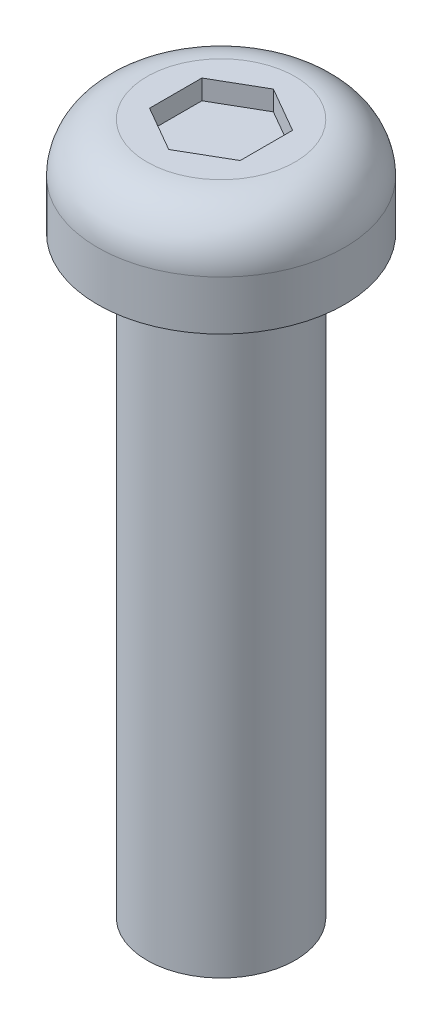
from build123d import *

# Parameters (mm, degrees)
SKETCH1_R           = 0.75
BOSS_EXTRUDE1_DEPTH = 6
SKETCH2_R           = 1.25
BOSS_EXTRUDE2_DEPTH = 1
FILLET1_R           = 0.5
CUT_EXTRUDE1_DEPTH  = 0.2


with BuildPart() as part:
    # Sketch1 → Boss-Extrude1 (new body)
    with BuildSketch(Plane(origin=(0, 0, 0), x_dir=(1, 0, 0), z_dir=(0, 1, 0))):
        with Locations(Location((0, 0, 0), (0, 0, 270))):
            Circle(SKETCH1_R)
    extrude(amount=BOSS_EXTRUDE1_DEPTH)

    # Sketch2 → Boss-Extrude2 (add)
    with BuildSketch(Plane(origin=(0, 6, 0), x_dir=(1, 0, 0), z_dir=(0, 1, 0))):
        with Locations(Location((0, 0, 0), (0, 0, 270))):
            Circle(SKETCH2_R)
    extrude(amount=BOSS_EXTRUDE2_DEPTH)

    # Fillet1
    fillet1_edges = [part.edges().sort_by_distance(p)[0] for p in [
        (0, 7, -1.25),
    ]]
    fillet(fillet1_edges, radius=FILLET1_R)

    # Sketch3 → Cut-Extrude1 (cut)
    with BuildSketch(Plane(origin=(0, 7, 0), x_dir=(1, 0, 0), z_dir=(0, 1, 0))):
        Polygon((0, 0.529895662), (-0.458903105, 0.264947831), (-0.458903105, -0.264947831), (0, -0.529895662), (0.458903105, -0.264947831), (0.458903105, 0.264947831), align=None)
    extrude(amount=-CUT_EXTRUDE1_DEPTH, mode=Mode.SUBTRACT)


solid = part.part
